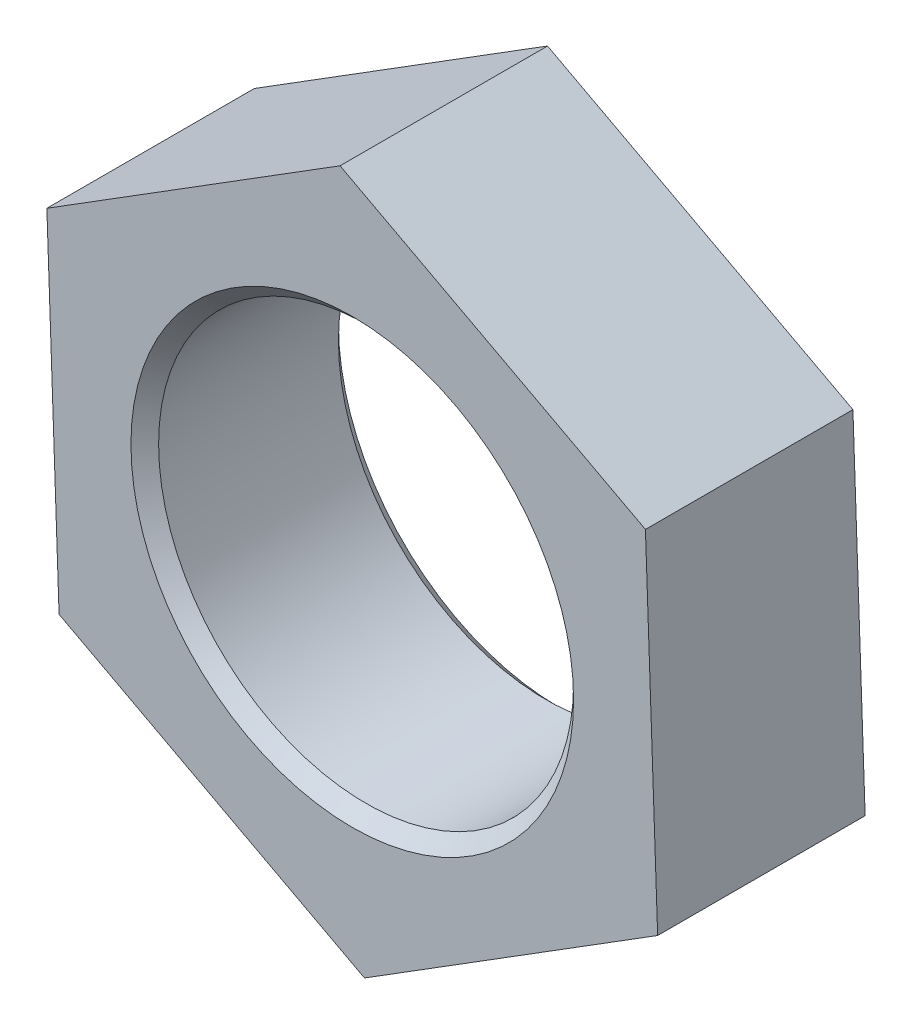
SolidWorks part; units mm, degrees
ref_plane "Front Plane" through (0, 0, 0) normal (0, 0, 1) x (1, 0, 0)
ref_plane "Top Plane" through (0, 0, 0) normal (0, 1, 0) x (1, 0, 0)
ref_plane "Right Plane" through (0, 0, 0) normal (1, 0, 0) x (0, 0, -1)
sketch "Sketch1" plane through (0, 0, 0) normal (0, 0, 1) x (1, 0, 0)
  line L1 (22.0787, -11.7273) -> (21.1955, 13.2571)
  line L2 (21.1955, 13.2571) -> (-0.8832, 24.9844)
  line L3 (-0.8832, 24.9844) -> (-22.0787, 11.7273)
  line L4 (-22.0787, 11.7273) -> (-21.1955, -13.2571)
  line L5 (-21.1955, -13.2571) -> (0.8832, -24.9844)
  line L6 (0.8832, -24.9844) -> (22.0787, -11.7273)
  circle A0 centre (0, 0) radius 15
  circle A1 centre (0, 0) radius 21.6506 construction
  dimension "D1" = 30
  dimension "D2" = 25
extrude "Boss-Extrude1" add sketch "Sketch1" along normal blind 15
cosmetic thread "Cosmetic Thread1" parameters "D2"=31
chamfer "Chamfer1" distance 1 angle 45 2 edges at (15, 0, 15) (15, 0, 0)
